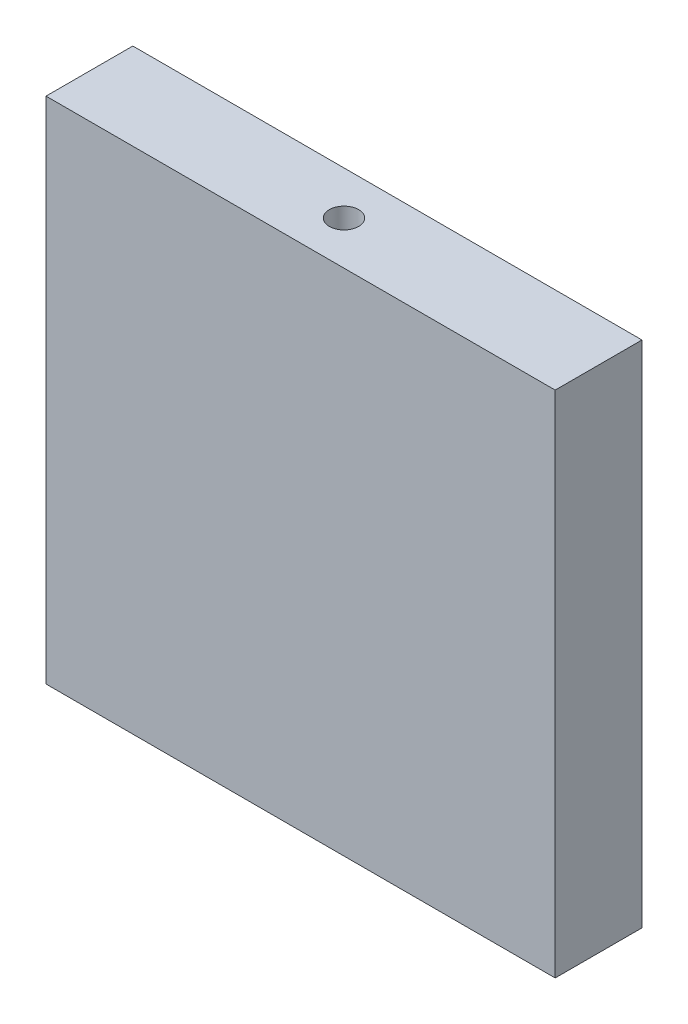
from build123d import *

# Parameters (mm, degrees)
SKETCH1_W           = 176
SKETCH1_H           = 176
BOSS_EXTRUDE1_DEPTH = 30
SKETCH3_R           = 5.055
CUT_EXTRUDE1_DEPTH  = 200.047732969


with BuildPart() as part:
    # Sketch1 → Boss-Extrude1 (new body)
    with BuildSketch(Plane.XY):
        Rectangle(SKETCH1_W, SKETCH1_H)
    extrude(amount=BOSS_EXTRUDE1_DEPTH)

    # Sketch3 → Cut-Extrude1 (cut, through all)
    with BuildSketch(Plane(origin=(0, 88, 0), x_dir=(1, 0, 0), z_dir=(0, 1, 0))):
        with Locations(Location((0, -15, 0), (0, 0, 180))):
            Circle(SKETCH3_R)
    extrude(amount=-CUT_EXTRUDE1_DEPTH, mode=Mode.SUBTRACT)


solid = part.part
